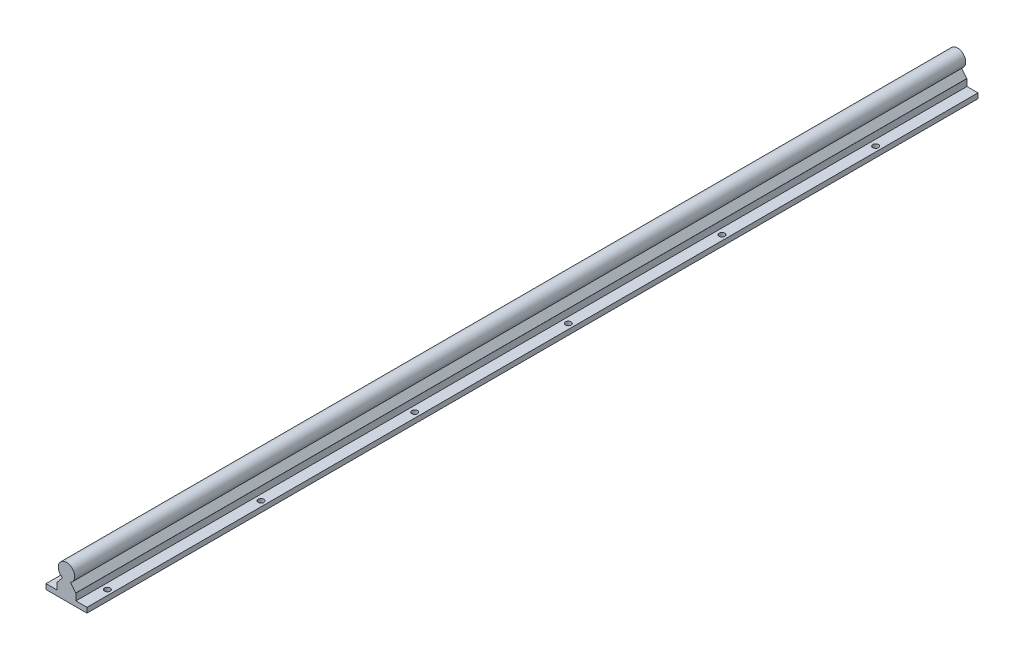
from build123d import *

# Parameters (mm, degrees)
EXTRUDE_1_DEPTH                  = 435
EXTRUDE_2_DEPTH                  = 870
HOLE_WIZARD_5_5_5_5_1_AT_2_COUNT = 2
HOLE_WIZARD_5_5_5_5_1_AT_2_PITCH = 30
PATTERN_LINEAR_1_COUNT           = 6
PATTERN_LINEAR_1_PITCH           = 150


with BuildPart() as part:
    # 草图1 → 凸台-拉伸1 (new, symmetric)
    with BuildSketch(Plane.XY):
        with BuildLine():
            Line((-9.25, 11.7), (-9.25, 5))
            Line((-9.25, 5), (-20, 5))
            Line((-20, 5), (-20, 0))
            Line((-20, 0), (20, 0))
            Line((20, 0), (20, 5))
            Line((20, 5), (9.25, 5))
            Line((9.25, 5), (9.25, 11.7))
            Line((9.25, 11.7), (9.11850775, 11.7))
            Line((9.11850775, 11.7), (4, 17.8))
            Line((4, 17.8), (3.487119155, 17.8))
            ThreePointArc((3.487119155, 17.8), (0, 17), (-3.487119155, 17.8))
            Line((-3.487119155, 17.8), (-4, 17.8))
            Line((-4, 17.8), (-9.11850775, 11.7))
            Line((-9.11850775, 11.7), (-9.25, 11.7))
        make_face()
    extrude(amount=EXTRUDE_1_DEPTH, both=True)

    # 草图2 → 凸台-拉伸2 (add)
    with BuildSketch(Plane.XY.offset(435)):
        with BuildLine():
            ThreePointArc((3.487119155, 17.8), (0, 33), (-3.487119155, 17.8))
            ThreePointArc((-3.487119155, 17.8), (0, 17), (3.487119155, 17.8))
        make_face()
    extrude(amount=-EXTRUDE_2_DEPTH)

    # 草图3 → Ø5.5 (5.5) 直径孔1 (revolve, cut)
    with BuildSketch(Plane(origin=(15, 5, 410), x_dir=(0, 0, 1), z_dir=(1, 0, 0))):
        Polygon((0, 0), (0, 17.19771324), (2.75, 15.61), (2.75, 0), align=None)
    hole_wizard_5_5_5_5_1 = revolve(axis=Axis((15, 11.35, 410), (0, -1, 0)), mode=Mode.SUBTRACT)

    # Ø5.5 (5.5) 直径孔1 at 2: Ø5.5 (5.5) 直径孔1 ×2
    with Locations(*[(-i * HOLE_WIZARD_5_5_5_5_1_AT_2_PITCH, 0, 0) for i in range(1, HOLE_WIZARD_5_5_5_5_1_AT_2_COUNT)]):
        add(hole_wizard_5_5_5_5_1, mode=Mode.SUBTRACT)

    # 阵列(线性)1: Ø5.5 (5.5) 直径孔1 ×6
    with Locations(*[(0, 0, -i * PATTERN_LINEAR_1_PITCH) for i in range(1, PATTERN_LINEAR_1_COUNT)]):
        add(hole_wizard_5_5_5_5_1, mode=Mode.SUBTRACT)

    # 阵列(线性)1 copy 1 sketch → 阵列(线性)1 copy 1 (revolve, cut)
    with BuildSketch(Plane(origin=(-15, 5, 260), x_dir=(0, 0, 1), z_dir=(1, 0, 0))):
        Polygon((0, 0), (0, 17.19771324), (2.75, 15.61), (2.75, 0), align=None)
    revolve(axis=Axis((-15, 11.35, 260), (0, -1, 0)), mode=Mode.SUBTRACT)

    # 阵列(线性)1 copy 2 sketch → 阵列(线性)1 copy 2 (revolve, cut)
    with BuildSketch(Plane(origin=(-15, 5, 110), x_dir=(0, 0, 1), z_dir=(1, 0, 0))):
        Polygon((0, 0), (0, 17.19771324), (2.75, 15.61), (2.75, 0), align=None)
    revolve(axis=Axis((-15, 11.35, 110), (0, -1, 0)), mode=Mode.SUBTRACT)

    # 阵列(线性)1 copy 3 sketch → 阵列(线性)1 copy 3 (revolve, cut)
    with BuildSketch(Plane(origin=(-15, 5, -40), x_dir=(0, 0, 1), z_dir=(1, 0, 0))):
        Polygon((0, 0), (0, 17.19771324), (2.75, 15.61), (2.75, 0), align=None)
    revolve(axis=Axis((-15, 11.35, -40), (0, -1, 0)), mode=Mode.SUBTRACT)

    # 阵列(线性)1 copy 4 sketch → 阵列(线性)1 copy 4 (revolve, cut)
    with BuildSketch(Plane(origin=(-15, 5, -190), x_dir=(0, 0, 1), z_dir=(1, 0, 0))):
        Polygon((0, 0), (0, 17.19771324), (2.75, 15.61), (2.75, 0), align=None)
    revolve(axis=Axis((-15, 11.35, -190), (0, -1, 0)), mode=Mode.SUBTRACT)

    # 阵列(线性)1 copy 5 sketch → 阵列(线性)1 copy 5 (revolve, cut)
    with BuildSketch(Plane(origin=(-15, 5, -340), x_dir=(0, 0, 1), z_dir=(1, 0, 0))):
        Polygon((0, 0), (0, 17.19771324), (2.75, 15.61), (2.75, 0), align=None)
    revolve(axis=Axis((-15, 11.35, -340), (0, -1, 0)), mode=Mode.SUBTRACT)


solid = part.part
